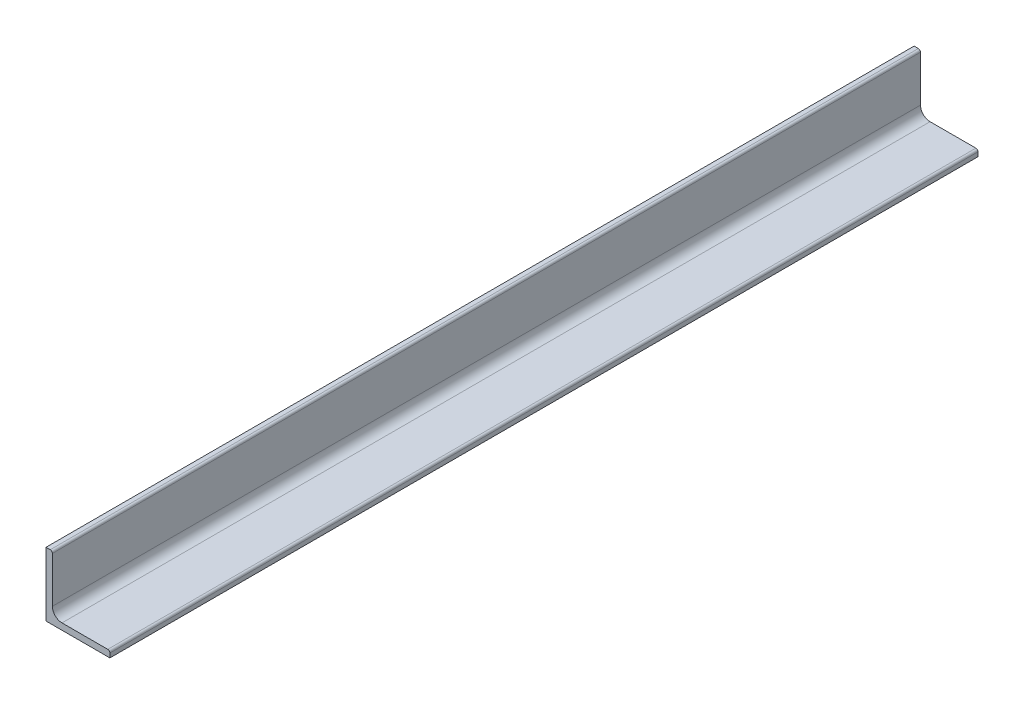
from build123d import *

# Parameters (mm, degrees)
BOSS_EXTRUDE1_DEPTH = 203.8


with BuildPart() as part:
    # Sketch1 → Boss-Extrude1 (new, symmetric)
    with BuildSketch(Plane.XY):
        with BuildLine():
            Line((0, 0), (0, 30))
            Line((0, 30), (2, 30))
            ThreePointArc((2, 30), (2.707106781, 29.707106781), (3, 29))
            Line((3, 29), (3, 7.5))
            ThreePointArc((3, 7.5), (4.318019485, 4.318019485), (7.5, 3))
            Line((7.5, 3), (29, 3))
            ThreePointArc((29, 3), (29.707106781, 2.707106781), (30, 2))
            Line((30, 2), (30, 0))
            Line((30, 0), (0, 0))
        make_face()
    extrude(amount=BOSS_EXTRUDE1_DEPTH, both=True)


solid = part.part
